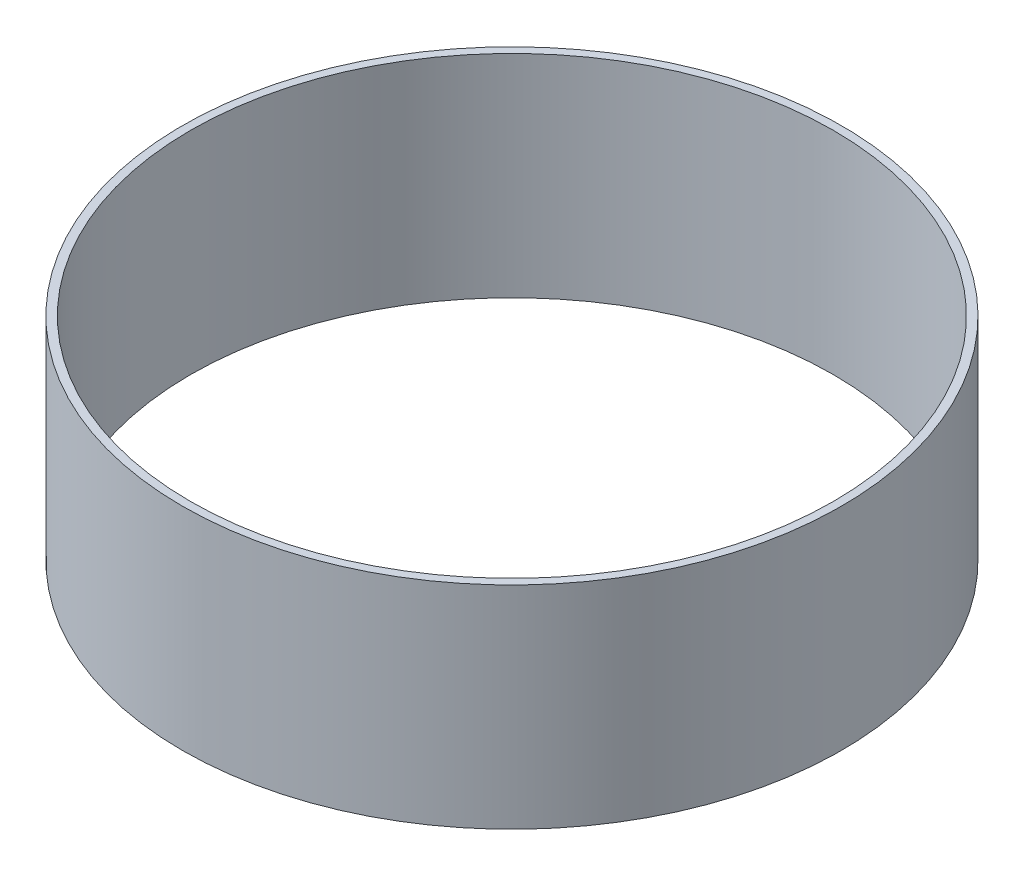
SolidWorks part; units mm, degrees
material "Q235B"
ref_plane "Front Plane" through (0, 0, 0) normal (0, 0, 1) x (1, 0, 0)
ref_plane "Top Plane" through (0, 0, 0) normal (0, 1, 0) x (1, 0, 0)
ref_plane "Right Plane" through (0, 0, 0) normal (1, 0, 0) x (0, 0, -1)
sketch "Sketch1" plane through (0, 0, 0) normal (0, 1, 0) x (1, 0, 0)
  circle A0 centre (0, 0) radius 405
  circle A1 centre (0, 0) radius 395
  dimension "D1" = 810
  dimension "D2" = 10
extrude "Boss-Extrude1" add sketch "Sketch1" along normal blind 260
